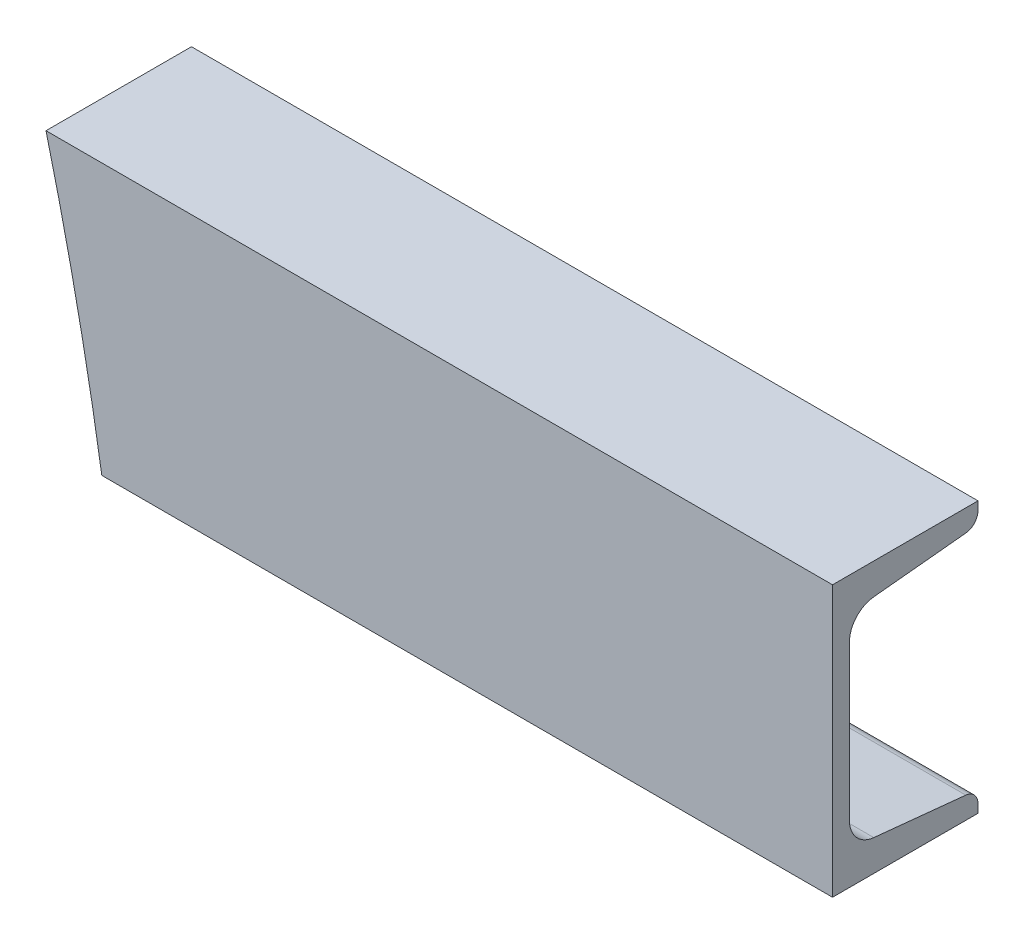
SolidWorks part; units mm, degrees
material "XRAAT"
ref_plane "前视基准面" through (0, 0, 0) normal (0, 0, 1) x (1, 0, 0)
ref_plane "上视基准面" through (0, 0, 0) normal (0, 1, 0) x (1, 0, 0)
ref_plane "右视基准面" through (0, 0, 0) normal (1, 0, 0) x (0, 0, -1)
sketch "草图1" plane through (0, 0, 0) normal (0, 0, 1) x (1, 0, 0)
  line L0 (0, 0) -> (300, 0)
  dimension "D1" = 300
other "热轧普通槽钢(gb t707-1988) 8-XXXXXXXXXXXXXXX528V9(1)"
ref_plane "基准面1" through (0, 0, 0) normal (-1, 0, 0) x (0, 0, -1)
sketch "Sketch11" plane through (0, 0, 0) normal (-1, 0, 0) x (0, 0, -1)
  line L0 (43, 80) -> (0, 80)
  line L1 (43, 0) -> (0, 0)
  line L2 (0, 80) -> (0, 0)
  line L3 (54.084, 120.3761) -> (64.084, 120.3761) construction
  line L4 (54.084, 120.3761) -> (54.084, 119.3761) construction
  line L5 (54.084, 119.3761) -> (64.084, 120.3761) construction
  line L6 (43, 80) -> (43, 77.52)
  line L7 (43, 0) -> (43, 2.48)
  line L8 (0, 40) -> (5, 40) construction
  line L9 (24, 72) -> (24, 80) construction
  line L10 (5, 62.8601) -> (5, 72) construction
  line L11 (5, 72) -> (43, 72) construction
  line L12 (5, 62.8601) -> (5, 17.1399)
  line L13 (43, 72) -> (43, 80) construction
  line L14 (43, 80) -> (43, 0) construction
  line L17 (12.204, 70.8204) -> (39.398, 73.5398)
  line L18 (12.204, 9.1796) -> (39.398, 6.4602)
  arc A0 (39.398, 73.5398) -> (43, 77.52) centre (39, 77.52) ccw
  arc A1 (39.398, 6.4602) -> (43, 2.48) centre (39, 2.48) cw
  arc A9 (5, 17.1399) -> (12.204, 9.1796) centre (13, 17.1399) ccw
  arc A10 (5, 62.8601) -> (12.204, 70.8204) centre (13, 62.8601) cw
  point P8 (0, 40)
  point P9 (5, 40)
  point P10 (21.5, 80)
  point P11 (21.5, 0)
  point P12 (43, 6.1)
  point P13 (43, 73.9)
  point P27 (43, 40)
  point P28 (0, 0)
  dimension "D4" = 43
  dimension "D5" = 5
  dimension "D2" = 10
  dimension "D8" = 8
  dimension "D3" = 80
  dimension "D6" = 8
  dimension "D7" = 4
  dimension "D1" = 1
sketch "草图4" plane through (0, 0, 0) normal (0, 0, 1) x (1, 0, 0)
  line L0 (67.5, 0) -> (300, 0)
  line L1 (0, 0) -> (300, 0) construction
  line L2 (84, -80) -> (300, -80)
  line L3 (300, -80) -> (0, -80) construction
  circle A0 centre (-799.8872, -220.6002) radius 895
  line M3 (0, 0) -> (0, -80)
  line M4 (0, -80) -> (300, -80)
  line M6 (300, 0) -> (0, 0)
  dimension "D1" = 1790
  dimension "D2" = 232.5
  dimension "D3" = 216
extrude "切除-拉伸2" cut sketch "草图4" against normal up to next contours A0 M4 M6 M3
sketch "草图5" [suppressed] plane through (0, 0, 0) normal (0, 0, 1) x (1, 0, 0)
  line L0 (84, 0) -> (300, 0)
  line L1 (300, 0) -> (0, 0) construction
  line L2 (300, -80) -> (67.5, -80)
  line L3 (300, -80) -> (0, -80) construction
  circle A0 centre (-799.8872, 140.6002) radius 895
  line M3 (0, 0) -> (0, -80)
  line M4 (0, -80) -> (300, -80)
  line M6 (300, 0) -> (0, 0)
  dimension "D1" = 1790
  dimension "D2" = 232.5
  dimension "D3" = 216
extrude "切除-拉伸3" [suppressed] cut sketch "草图5" against normal up to next contours A0 M4 M6 M3
